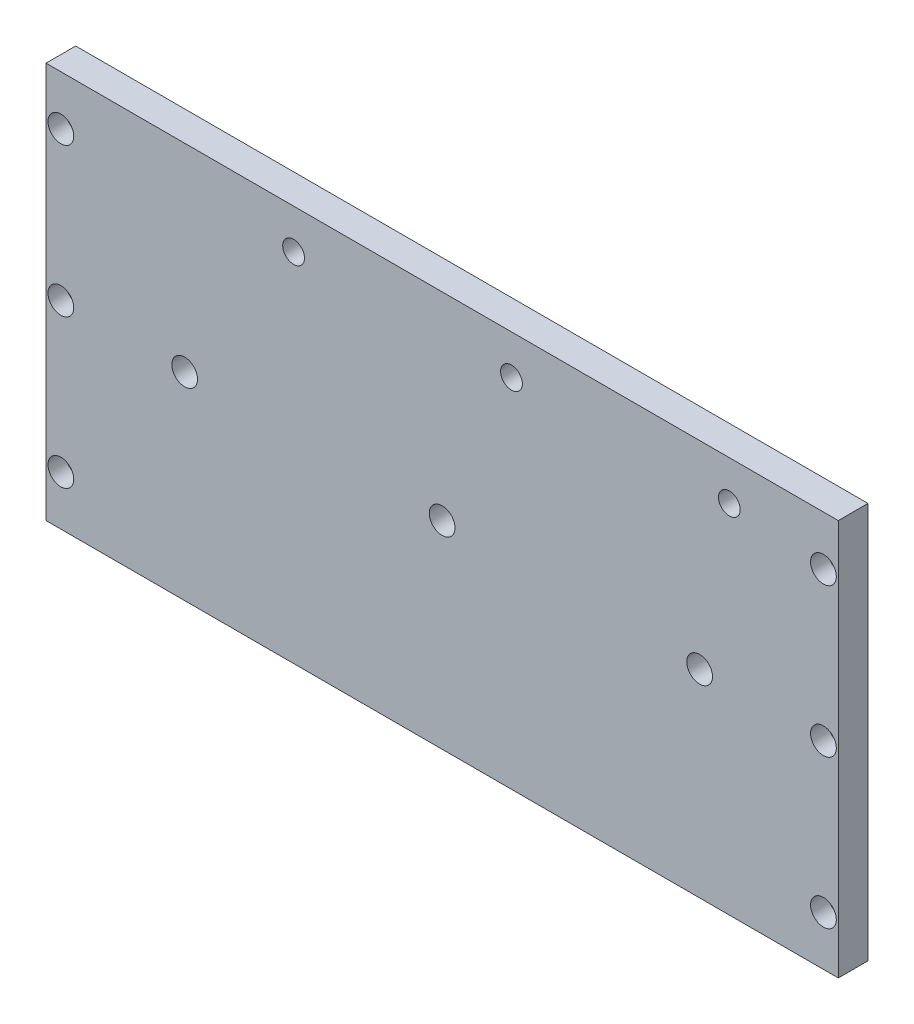
SolidWorks part; units mm, degrees
ref_plane "Front Plane" through (0, 0, 0) normal (0, 0, 1) x (1, 0, 0)
ref_plane "Top Plane" through (0, 0, 0) normal (0, 1, 0) x (1, 0, 0)
ref_plane "Right Plane" through (0, 0, 0) normal (1, 0, 0) x (0, 0, -1)
sketch "Sketch1" plane through (0, 0, 0) normal (0, 0, 1) x (1, 0, 0)
  line L1 (200, -100) -> (-200, -100)
  line L2 (200, -100) -> (200, 100)
  line L3 (200, 100) -> (-200, 100)
  line L4 (-200, -100) -> (-200, 100)
  line L5 (200, -100) -> (-200, 100) construction
  line L6 (200, 100) -> (-200, -100) construction
  point P1 (0, 0)
  dimension "D1" = 400
  dimension "D2" = 200
extrude "Boss-Extrude1" add sketch "Sketch1" along normal blind 15
sketch "Sketch2" plane through (0, 0, 15) normal (0, 0, 1) x (1, 0, 0)
  circle A0 centre (-192.5, 75) radius 6.5
  dimension "D1" = 13
extrude "Cut-Extrude1" cut sketch "Sketch2" against normal blind 9
pattern_linear "LPattern1" count 3 spacing 75 along (0, -1, 0) of "Cut-Extrude1"
mirror "Mirror1" about plane through (0, 0, 0) normal (1, 0, 0) of "LPattern1", "Cut-Extrude1"
sketch "Sketch3" plane through (0, 0, 15) normal (0, 0, 1) x (1, 0, 0)
  circle A0 centre (-192.5, 75) radius 4.5
  dimension "D1" = 9
extrude "Cut-Extrude2" cut sketch "Sketch3" against normal blind 85
pattern_linear "LPattern2" count 3 spacing 75 along (0, -1, 0) of "Cut-Extrude2"
mirror "Mirror2" about plane through (0, 0, 0) normal (1, 0, 0) of "LPattern2", "Cut-Extrude2"
sketch "Sketch4" plane through (0, 0, 15) normal (0, 0, 1) x (1, 0, 0)
  line L0 (8.25, 0) -> (-8.25, 0) construction
  line L1 (0, -8.25) -> (0, 8.25) construction
  circle A0 centre (-130, 0) radius 6.5
  dimension "D1" = 13
  dimension "D2" = 130
extrude "Cut-Extrude3" cut sketch "Sketch4" against normal blind 85
pattern_linear "LPattern3" count 3 spacing 130 along (1, 0, 0) of "Cut-Extrude3"
sketch "Sketch5" plane through (0, 0, 15) normal (0, 0, 1) x (1, 0, 0)
  line L0 (200, 100) -> (-200, 100) construction
  line L1 (0, -8.25) -> (0, 8.25) construction
  circle A0 centre (-75, 80) radius 5.5
  dimension "D1" = 11
  dimension "D2" = 20
  dimension "D3" = 75
extrude "Cut-Extrude4" cut sketch "Sketch5" against normal blind 51
pattern_linear "LPattern4" count 3 spacing 110 along (1, 0, 0) of "Cut-Extrude4"
